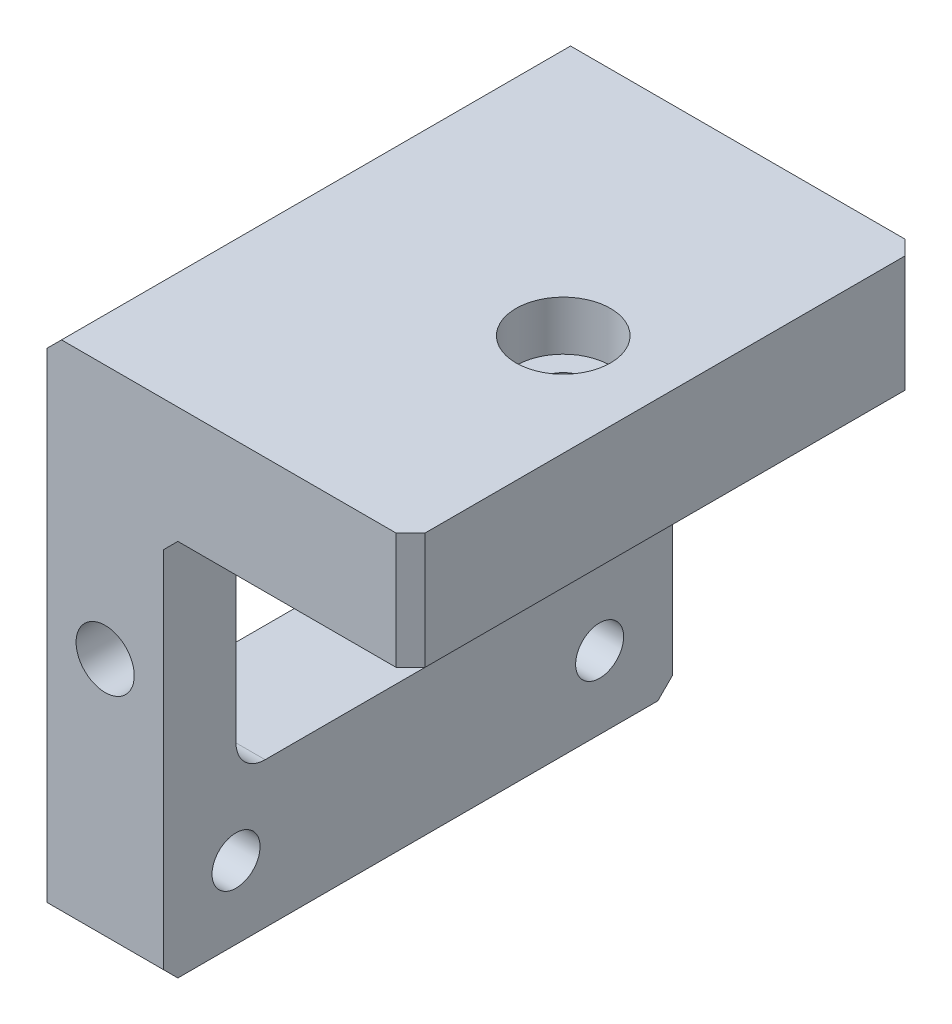
SolidWorks part; units mm, degrees
material "S45C"
ref_plane "Front Plane" through (0, 0, 0) normal (0, 0, 1) x (1, 0, 0)
ref_plane "Top Plane" through (0, 0, 0) normal (0, 1, 0) x (1, 0, 0)
ref_plane "Right Plane" through (0, 0, 0) normal (1, 0, 0) x (0, 0, -1)
sketch "Sketch1" plane through (0, 0, 0) normal (0, 0, 1) x (1, 0, 0)
  line L0 (0, 0) -> (0, 35)
  line L1 (0, 35) -> (25, 35)
  line L2 (25, 35) -> (25, 27)
  line L3 (25, 27) -> (8, 27)
  line L4 (8, 27) -> (8, 0)
  line L5 (8, 0) -> (0, 0)
  dimension "D1" = 35
  dimension "D2" = 8
  dimension "D3" = 8
  dimension "D4" = 25
extrude "Boss-Extrude1" add sketch "Sketch1" along normal mid plane 35
sketch "Sketch2" plane through (0, 0, 0) normal (-1, 0, 0) x (0, 0, 1)
  line L2 (-12.5, 25) -> (12.5, 25)
  line L3 (-12.5, 25) -> (-12.5, 10)
  line L4 (-12.5, 10) -> (12.5, 10)
  line L5 (12.5, 25) -> (12.5, 10)
  line L6 (0, 10) -> (0, 0) construction
  line L7 (17.5, 0) -> (-17.5, 0) construction
  dimension "D1" = 10
  dimension "D2" = 15
  dimension "D3" = 25
extrude "Cut-Extrude1" cut sketch "Sketch2" against normal through all
hole_wizard "M4 Tapped Hole1" positions "Sketch4" profile "Sketch3" tap size "M4" standard "GB"
sketch "Sketch4" plane through (0, 0, 0) normal (-1, 0, 0) x (0, 0, 1)
  line L0 (-12.5, 5) -> (12.5, 5) construction
  line L3 (0, 5) -> (0, 0) construction
  line L5 (17.5, 0) -> (-17.5, 0) construction
  point P0 (-12.5, 5)
  point P1 (12.5, 5)
  dimension "D1" = 25
  dimension "D2" = 5
sketch "Sketch3" plane through (0, 5, -12.5) normal (0, 1, 0) x (0, 0, 1)
  line L0 (0, 0) -> (0, 12.4914)
  line L1 (0, 12.4914) -> (1.65, 11.5)
  line L2 (1.65, 11.5) -> (1.65, 0)
  line L5 (1.65, 0) -> (0, 0)
  line L10 (0, 12.4914) -> (-1.65, 11.5) construction
  line L11 (0, -6.35) -> (0, 107.95) construction
  dimension "螺纹孔钻头直径" = 3.3
  dimension "螺纹孔钻头深度" = 11.5
  dimension "导头角度" = 118
cosmetic thread "Cosmetic Thread 1" parameters "D1"=8, "D2"=4
cosmetic thread "Cosmetic Thread 2" parameters "D1"=8, "D2"=4
sketch "Sketch5" plane through (0, 0, 17.5) normal (0, 0, 1) x (1, 0, 0)
  line L0 (4, 17.5) -> (4, 0) construction
  line L1 (0, 0) -> (8, 0) construction
  circle A0 centre (4, 17.5) radius 2
  dimension "D1" = 17.5
  dimension "D2" = 4
extrude "Cut-Extrude2" cut sketch "Sketch5" against normal through all
fillet "Fillet1" radius 2 4 edges at (4, 10, -12.5) (4, 10, 12.5) (4, 25, 12.5) (4, 25, -12.5)
sketch "Sketch6" plane through (0, 27, 0) normal (0, -1, 0) x (1, 0, 0)
  line L0 (0, 17.5) -> (0, -17.5) construction
  circle A0 centre (18, 0) radius 4
  dimension "D1" = 8
  dimension "D2" = 18
extrude "Cut-Extrude3" cut sketch "Sketch6" against normal blind 3
chamfer "Chamfer1" distance 1 angle 45 6 edges at (8, 27, 0) (4, 0, -17.5) (4, 0, 17.5) (0, 35, 0) (25, 31, 17.5) (25, 31, -17.5)
hole_wizard "CBORE for M3 Hex Socket Head Cap Screw1" positions "Sketch8" profile "Sketch7" counterbore size "M3" standard "Iso" end condition through all
sketch "Sketch8" plane through (0, 35, 0) normal (0, 1, 0) x (1, 0, 0)
  line L0 (25, 0) -> (0, 0) construction
  line L1 (25, -16.5) -> (25, 16.5) construction
  line L3 (0, -17.5) -> (0, 17.5) construction
  point P0 (18, 0)
  dimension "D1" = 18
sketch "Sketch7" plane through (18, 35, 0) normal (1, 0, 0) x (0, 0, 1)
  line L0 (0, 0) -> (0, 35)
  line L1 (0, 35) -> (1.7, 35)
  line L3 (1.7, 35) -> (1.7, 3.4)
  line L4 (1.7, 3.4) -> (3.25, 3.4)
  line L5 (3.25, 3.4) -> (3.25, 0)
  line L7 (3.25, 0) -> (0, 0)
  line L11 (0, -6.35) -> (0, 107.95) construction
  dimension "通孔孔直径" = 3.4
  dimension "通孔孔深度" = 35
  dimension "柱形沉头孔直径" = 6.5
  dimension "柱形沉头孔深度" = 3.4
